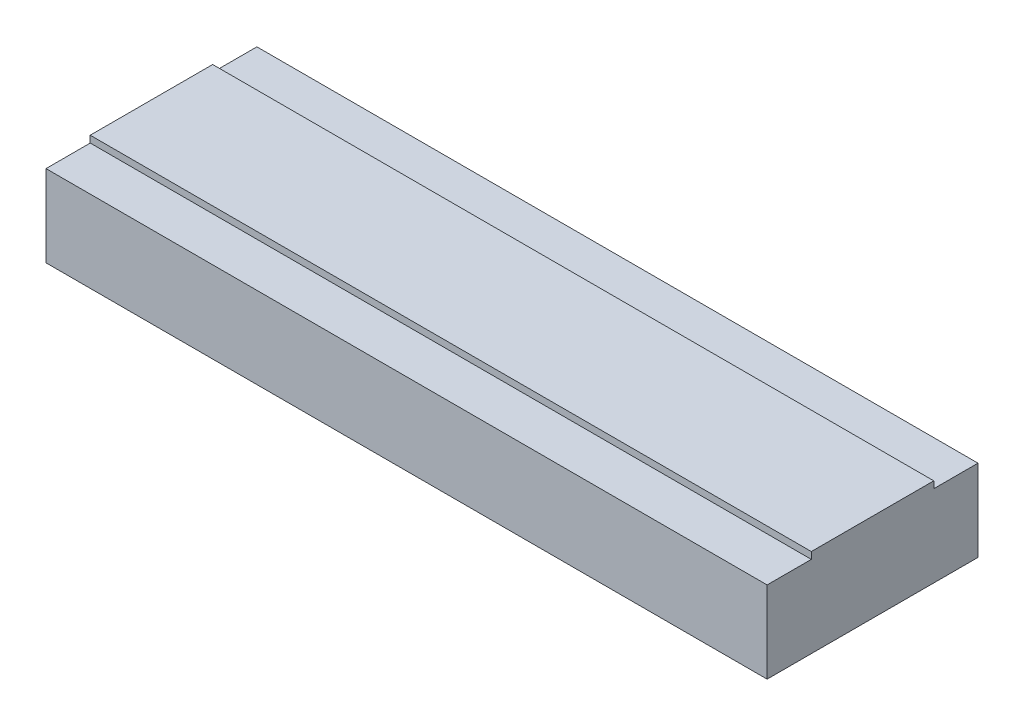
SolidWorks part; units mm, degrees
ref_plane "Front Plane" through (0, 0, 0) normal (0, 0, 1) x (1, 0, 0)
ref_plane "Top Plane" through (0, 0, 0) normal (0, 1, 0) x (1, 0, 0)
ref_plane "Right Plane" through (0, 0, 0) normal (1, 0, 0) x (0, 0, -1)
sketch "Sketch1" plane through (0, 0, 0) normal (0, 1, 0) x (1, 0, 0)
  line L1 (-106, -31) -> (106, -31)
  line L2 (-106, -31) -> (-106, 31)
  line L3 (-106, 31) -> (106, 31)
  line L4 (106, -31) -> (106, 31)
  line L5 (-106, -31) -> (106, 31) construction
  line L6 (-106, 31) -> (106, -31) construction
  point P0 (0, 0)
  dimension "D1" = 212
  dimension "D2" = 62
extrude "Boss-Extrude1" add sketch "Sketch1" along normal blind 26
sketch "Sketch2" plane through (106, 0, 0) normal (1, 0, 0) x (0, 0, -1)
  line L0 (31, 24) -> (18, 24)
  line L1 (31, 26) -> (31, 0) construction
  line L2 (18, 24) -> (18, 26)
  line L3 (-31, 26) -> (31, 26) construction
  line L4 (18, 26) -> (31, 26)
  line L5 (31, 26) -> (31, 24)
  line L6 (0, 14.3) -> (0, -14.3) construction
  line L7 (0, 26) -> (0, 6.8255) construction
  line L8 (-31, 26) -> (-31, 24)
  line L9 (-18, 26) -> (-31, 26)
  line L10 (-18, 24) -> (-18, 26)
  line L11 (-31, 24) -> (-18, 24)
  dimension "D1" = 18
  dimension "D2" = 2
shell "Shell1" thickness 7.5
extrude "Cut-Extrude2" cut sketch "Sketch2" against normal through all contours L0 L2 L4 L5 | L11 L10 L9 L8
sketch "Sketch3" plane through (0, 0, 0) normal (0, -1, 0) x (1, 0, 0)
  line L0 (45.5, 23.5) -> (45.5, -23.5)
  line L1 (-98.5, 23.5) -> (98.5, 23.5) construction
  line L2 (98.5, -23.5) -> (-98.5, -23.5) construction
  line L3 (98.5, 23.5) -> (98.5, -23.5) construction
  line L4 (-45.5, 23.516) -> (-45.5, -23.5)
  line L5 (98.5, -23.5) -> (-98.5, -23.5) construction
  line L6 (-98.5, -23.5) -> (-98.5, 23.5) construction
  dimension "D1" = 53
  dimension "D2" = 53
rib "Rib1" sketch "Sketch3" sketch "Sketch3" thickness 6 extrusion direction normal to sketch draft on no parameters "D1"=6
sketch "Sketch4" plane through (0, 0, 0) normal (0, -1, 0) x (1, 0, 0)
  line L0 (86.5, 23.5) -> (98.5, 11.5)
  line L1 (48.5, 23.5) -> (98.5, 23.5) construction
  line L2 (98.5, 23.5) -> (98.5, -23.5) construction
  line L3 (98.5, 11.5) -> (98.5, 23.5)
  line L4 (98.5, 23.5) -> (86.5, 23.5)
  line L5 (-98.5, -11.5) -> (-86.5, -23.5)
  line L6 (-98.5, -23.5) -> (-98.5, 23.5) construction
  line L7 (-48.5, -23.5) -> (-98.5, -23.5) construction
  line L8 (-86.5, -23.5) -> (-98.5, -23.5)
  line L9 (-98.5, -23.5) -> (-98.5, -11.5)
  dimension "D1" = 12
  dimension "D2" = 12
  dimension "D3" = 12
  dimension "D4" = 12
extrude "Boss-Extrude2" add sketch "Sketch4" against normal up to next
